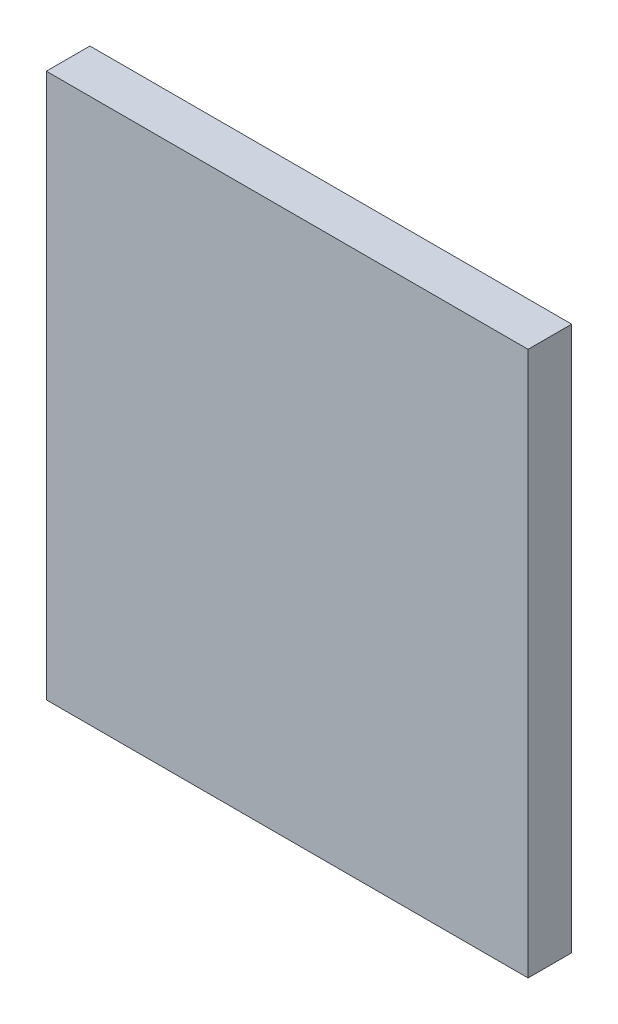
SolidWorks part; units mm, degrees
ref_plane "Front Plane" through (0, 0, 0) normal (0, 0, 1) x (1, 0, 0)
ref_plane "Top Plane" through (0, 0, 0) normal (0, 1, 0) x (1, 0, 0)
ref_plane "Right Plane" through (0, 0, 0) normal (1, 0, 0) x (0, 0, -1)
sketch "Sketch1" plane through (0, 0, 0) normal (0, 0, 1) x (1, 0, 0)
  line L1 (-55.984, 63.789) -> (54.5032, 63.789)
  line L2 (-55.984, 63.789) -> (-55.984, -61.0789)
  line L3 (-55.984, -61.0789) -> (54.5032, -61.0789)
  line L4 (54.5032, 63.789) -> (54.5032, -61.0789)
extrude "Boss-Extrude1" add sketch "Sketch1" along normal blind 10
